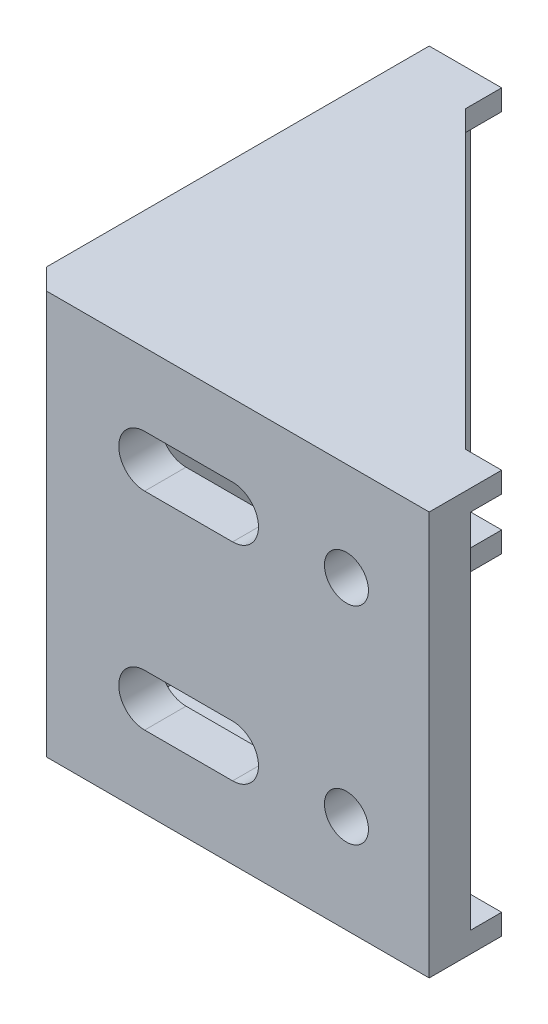
SolidWorks part; units mm, degrees
ref_plane "Front Plane" through (0, 0, 0) normal (0, 0, 1) x (1, 0, 0)
ref_plane "Top Plane" through (0, 0, 0) normal (0, 1, 0) x (1, 0, 0)
ref_plane "Right Plane" through (0, 0, 0) normal (1, 0, 0) x (0, 0, -1)
ref_plane "Plane1" through (0, 78, 0) normal (0, 1, 0) x (1, 0, 0)
sketch "Sketch1" plane through (0, 78, 0) normal (0, 1, 0) x (1, 0, 0)
  line L0 (-19.7308, -49.5782) -> (37.2692, -49.5782)
  line L1 (37.2692, -49.5782) -> (-19.7308, 7.4218)
  line L2 (-19.7308, 7.4218) -> (-19.7308, -49.5782)
extrude "Boss-Extrude1" add sketch "Sketch1" against normal blind 74
sketch "Sketch2" plane through (0, 0, 49.5782) normal (0, 0, 1) x (1, 0, 0)
  line L0 (-19.7308, 4) -> (-19.7308, 78)
  line L1 (-19.7308, 78) -> (44.2692, 78)
  line L2 (44.2692, 78) -> (44.2692, 4)
  line L3 (44.2692, 4) -> (-19.7308, 4)
extrude "Boss-Extrude2" add sketch "Sketch2" along normal blind 14
sketch "Sketch3" plane through (0, 4, 0) normal (0, -1, 0) x (1, 0, 0)
  line L0 (-19.7308, 63.5782) -> (44.2692, 63.5782)
  line L1 (44.2692, 63.5782) -> (44.2692, -14.4218)
  line L2 (44.2692, -14.4218) -> (-19.7308, -14.4218)
  line L3 (-19.7308, -14.4218) -> (-19.7308, 63.5782)
extrude "Boss-Extrude3" add sketch "Sketch3" along normal blind 4
ref_plane "Plane2" through (0, 4, 0) normal (0, -1, 0) x (1, 0, 0)
sketch "Sketch4" plane through (0, 4, 0) normal (0, -1, 0) x (1, 0, 0)
  line L0 (-19.7308, -7.4218) -> (37.2692, 49.5782)
  line L1 (37.2692, 49.5782) -> (-19.7308, 49.5782)
  line L2 (-19.7308, 49.5782) -> (-19.7308, -7.4218)
extrude "Cut-Extrude1" cut sketch "Sketch4" against normal blind 70
sketch "Sketch5" plane through (-19.7308, 0, 0) normal (-1, 0, 0) x (0, 0, 1)
  line L0 (63.5782, 0) -> (-14.4218, 0)
  line L1 (-14.4218, 0) -> (-14.4218, 78)
  line L2 (-14.4218, 78) -> (63.5782, 78)
  line L3 (63.5782, 78) -> (63.5782, 0)
extrude "Boss-Extrude4" add sketch "Sketch5" along normal blind 14
ref_plane "Plane3" through (0, 0, 49.5782) normal (0, 0, -1) x (-1, 0, 0)
ref_plane "Plane4" through (0, 0, 55.5782) normal (0, 0, 1) x (1, 0, 0)
sketch "Sketch7" plane through (0, 0, 55.5782) normal (0, 0, 1) x (1, 0, 0)
  line L0 (-19.7308, 74) -> (-19.7308, 4)
  line L1 (-19.7308, 4) -> (44.2692, 4)
  line L2 (44.2692, 4) -> (44.2692, 74)
  line L3 (44.2692, 74) -> (-19.7308, 74)
extrude "Cut-Extrude2" cut sketch "Sketch7" against normal up to surface up to plane "Plane3"
ref_plane "Plane5" through (-19.7308, 0, 0) normal (1, 0, 0) x (0, 0, -1)
ref_plane "Plane6" through (-25.7308, 0, 0) normal (-1, 0, 0) x (0, -1, 0)
sketch "Sketch9" plane through (-25.7308, 0, 0) normal (-1, 0, 0) x (0, -1, 0)
  line L0 (-4, 55.5782) -> (-74, 55.5782)
  line L1 (-74, 55.5782) -> (-74, -14.4218)
  line L2 (-74, -14.4218) -> (-4, -14.4218)
  line L3 (-4, -14.4218) -> (-4, 55.5782)
extrude "Cut-Extrude3" cut sketch "Sketch9" against normal up to surface up to plane "Plane5"
sketch "Sketch10" plane through (0, 0, 0) normal (0, -1, 0) x (1, 0, 0)
  line L0 (44.2692, 49.5782) -> (37.2692, 49.5782)
  line L1 (37.2692, 49.5782) -> (-19.7308, -7.4218)
  line L2 (-19.7308, -7.4218) -> (-19.7308, -14.4218)
  line L3 (-19.7308, -14.4218) -> (44.2692, -14.4218)
  line L4 (44.2692, -14.4218) -> (44.2692, 49.5782)
extrude "Cut-Extrude4" cut sketch "Sketch10" against normal through all
sketch "Sketch11" plane through (-25.7308, 0, 0) normal (1, 0, 0) x (0, 0, -1)
  line L0 (-23.5782, 24) -> (-40.5782, 24)
  line L1 (-40.5782, 14) -> (-23.5782, 14)
  arc A0 (-40.5782, 24) -> (-40.5782, 14) centre (-40.5782, 19) ccw
  arc A1 (-23.5782, 14) -> (-23.5782, 24) centre (-23.5782, 19) ccw
extrude "Cut-Extrude5" cut sketch "Sketch11" against normal through all
sketch "Sketch12" plane through (0, 0, 63.5782) normal (0, 0, 1) x (1, 0, 0)
  line L0 (6.2692, 64) -> (-10.7308, 64)
  line L1 (-10.7308, 54) -> (6.2692, 54)
  arc A0 (-10.7308, 64) -> (-10.7308, 54) centre (-10.7308, 59) ccw
  arc A1 (6.2692, 54) -> (6.2692, 64) centre (6.2692, 59) ccw
extrude "Cut-Extrude6" cut sketch "Sketch12" against normal through all
sketch "Sketch13" plane through (0, 0, 63.5782) normal (0, 0, 1) x (1, 0, 0)
  line L0 (6.2692, 24) -> (-10.7308, 24)
  line L1 (-10.7308, 14) -> (6.2692, 14)
  arc A0 (-10.7308, 24) -> (-10.7308, 14) centre (-10.7308, 19) ccw
  arc A1 (6.2692, 14) -> (6.2692, 24) centre (6.2692, 19) ccw
extrude "Cut-Extrude7" cut sketch "Sketch13" against normal through all
sketch "Sketch14" plane through (-33.7308, 0, 0) normal (-1, 0, 0) x (0, 0, 1)
  line L0 (23.0782, 54) -> (40.0782, 54)
  line L1 (40.0782, 64) -> (23.0782, 64)
  arc A0 (40.0782, 54) -> (40.0782, 64) centre (40.0782, 59) ccw
  arc A1 (23.0782, 64) -> (23.0782, 54) centre (23.0782, 59) ccw
extrude "Cut-Extrude8" cut sketch "Sketch14" against normal through all
hole_wizard "Ø8.5 (8.5) Diameter Hole1" positions "Sketch16" profile "Sketch15" hole size "Ø8.5" standard "ANSI Metric"
sketch "Sketch16" plane through (-33.7308, 0, 0) normal (-1, 0, 0) x (0, 0, 1)
  point P0 (1.5782, 59)
  point P1 (1.5782, 19)
sketch "Sketch15" plane through (-33.7308, 59, 1.5782) normal (0, 1, 0) x (0, 0, 1)
  line L0 (0, 0) -> (0, 78)
  line L1 (0, 78) -> (4.25, 78)
  line L2 (4.25, 78) -> (4.25, 0)
  line L5 (4.25, 0) -> (0, 0)
  line L11 (0, -6.35) -> (0, 107.95) construction
  dimension "通孔孔直径" = 8.5
  dimension "通孔孔深度" = 78
hole_wizard "Ø8.5 (8.5) Diameter Hole2" positions "Sketch18" profile "Sketch17" hole size "Ø8.5" standard "ANSI Metric"
sketch "Sketch18" plane through (0, 0, 63.5782) normal (0, 0, 1) x (1, 0, 0)
  point P0 (28.2692, 19)
  point P1 (28.2692, 59)
sketch "Sketch17" plane through (28.2692, 19, 63.5782) normal (1, 0, 0) x (0, -1, 0)
  line L0 (0, 0) -> (0, 78)
  line L1 (0, 78) -> (4.25, 78)
  line L2 (4.25, 78) -> (4.25, 0)
  line L5 (4.25, 0) -> (0, 0)
  line L11 (0, -6.35) -> (0, 107.95) construction
  dimension "通孔孔直径" = 8.5
  dimension "通孔孔深度" = 78
chamfer "Chamfer1" distance 4 angle 45 1 edges at (-33.7308, 39, 63.5782)
